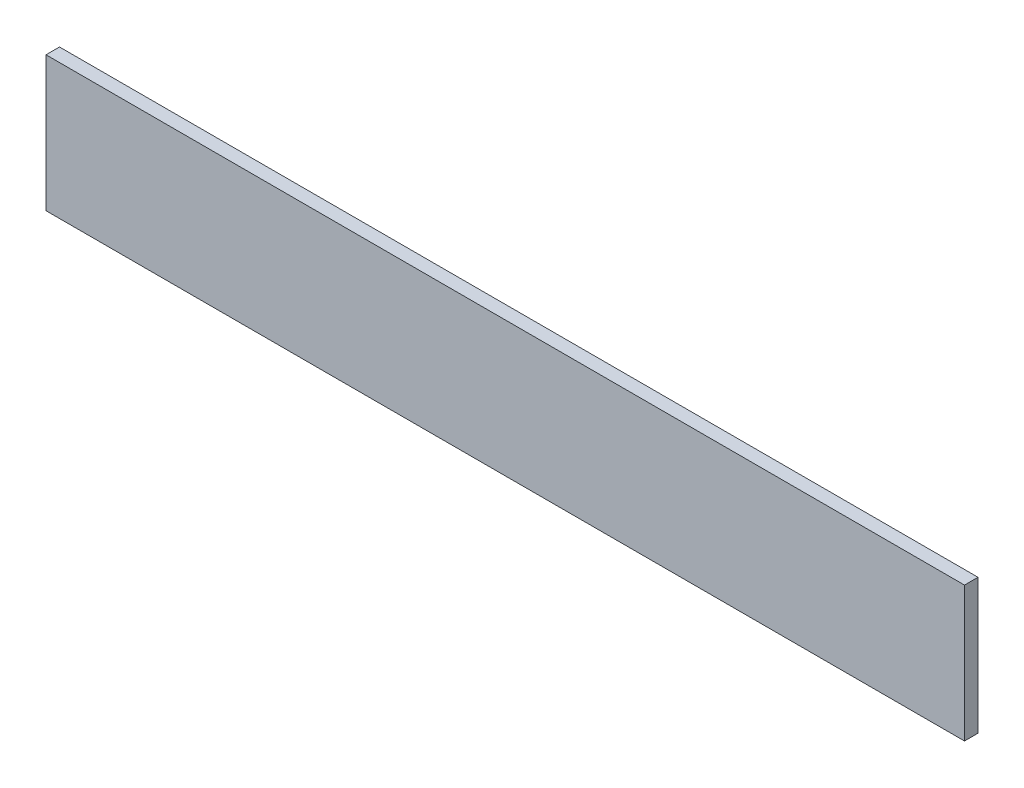
from build123d import *

# Parameters (mm, degrees)
SKETCH_1_W      = 340
SKETCH_1_H      = 50
EXTRUDE_1_DEPTH = 5


with BuildPart() as part:
    # 草图1 → 凸台-拉伸1 (new body)
    with BuildSketch(Plane.XY):
        with Locations((170, 25)):
            Rectangle(SKETCH_1_W, SKETCH_1_H)
    extrude(amount=EXTRUDE_1_DEPTH)


solid = part.part
